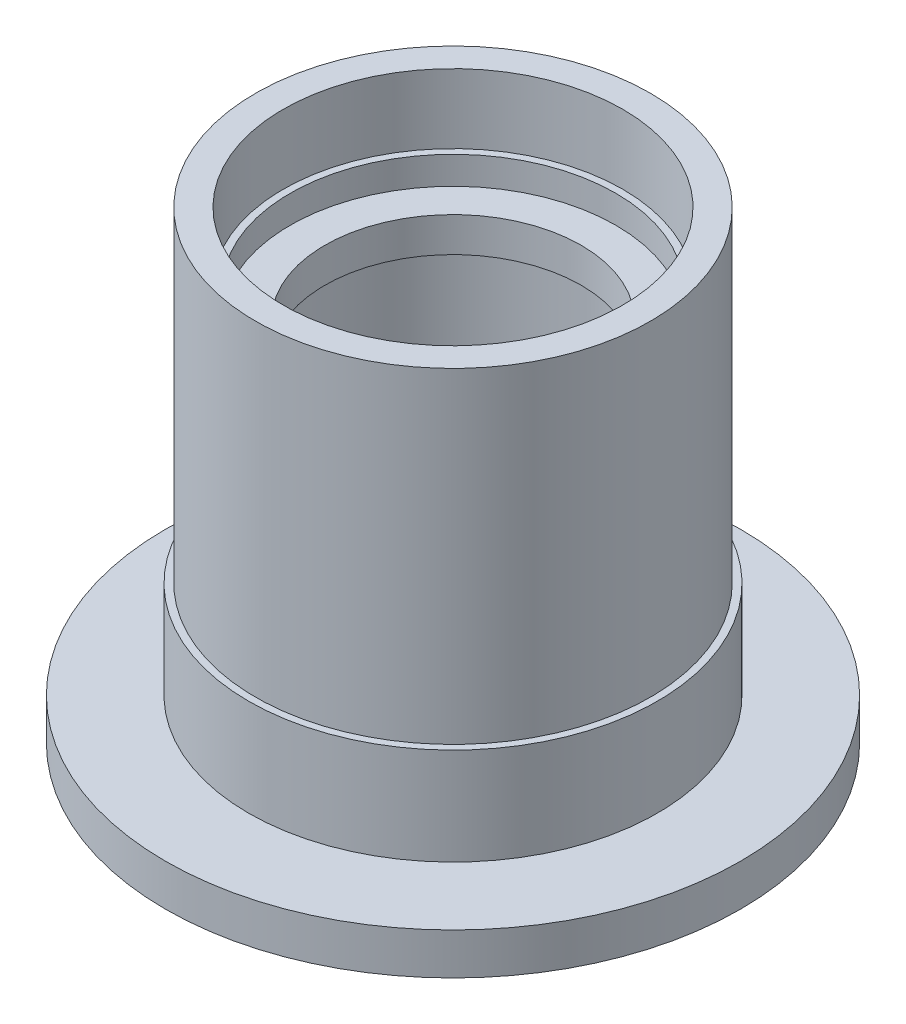
SolidWorks part; units mm, degrees
ref_plane "前视基准面" through (0, 0, 0) normal (0, 0, 1) x (1, 0, 0)
ref_plane "上视基准面" through (0, 0, 0) normal (0, 1, 0) x (1, 0, 0)
ref_plane "右视基准面" through (0, 0, 0) normal (1, 0, 0) x (0, 0, -1)
sketch "草图1" plane through (0, 0, 0) normal (0, 0, 1) x (1, 0, 0)
  line L1 (-23.5, 57) -> (-23.5, 53)
  line L2 (-23.5, 53) -> (-18.5, 53)
  line L4 (-21.5, 24) -> (-23.5, 24)
  line L5 (-23.5, 24) -> (-23.5, 0)
  line L6 (-23.5, 0) -> (-41.5, 0)
  line L7 (-28.5, 67) -> (-28.5, 20)
  line L8 (-28.5, 20) -> (-29.5, 20)
  line L9 (-29.5, 20) -> (-29.5, 6)
  line L10 (-29.5, 6) -> (-41.5, 6)
  line L11 (-41.5, 6) -> (-41.5, 0)
  line L12 (-23.5, 57) -> (-24.5, 57)
  line L13 (-24.5, 57) -> (-24.5, 67)
  line L14 (-24.5, 67) -> (-28.5, 67)
  line L15 (0, 0) -> (0, 61.9675) construction
  line L16 (-18.5, 53) -> (-18.5, 48)
  line L17 (-18.5, 48) -> (-21.5, 48)
  line L18 (-21.5, 48) -> (-21.5, 24)
  dimension "D1" = 24
  dimension "D2" = 23.5
  dimension "D3" = 2
  dimension "D4" = 4
  dimension "D5" = 29
  dimension "D6" = 1
  dimension "D7" = 10
  dimension "D8" = 14
  dimension "D9" = 1
  dimension "D10" = 5
  dimension "D11" = 6
  dimension "D12" = 12
  dimension "D13" = 5
  dimension "D14" = 7
revolve "旋转1" add sketch "草图1" angle 360 about L15
sketch "草图2" plane through (0, 0, 0) normal (0, -1, 0) x (1, 0, 0)
  circle A0 centre (0, 0) radius 29.5
  circle A1 centre (0, 0) radius 23.5 construction
  circle A2 centre (0, 0) radius 23.5
  dimension "D1" = 59
extrude "凸台-拉伸1" [suppressed] add sketch "草图2" along normal blind 2
